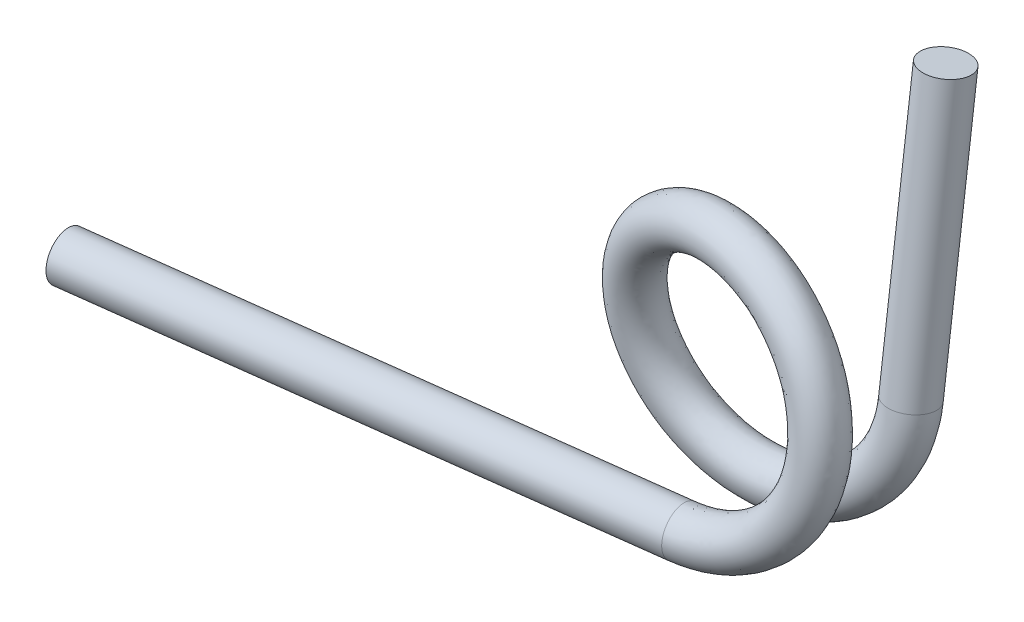
SolidWorks part; units mm, degrees
ref_plane "Front Plane" through (0, 0, 0) normal (0, 0, 1) x (1, 0, 0)
ref_plane "Top Plane" through (0, 0, 0) normal (0, 1, 0) x (1, 0, 0)
ref_plane "Right Plane" through (0, 0, 0) normal (1, 0, 0) x (0, 0, -1)
other "Configuration Table"
sketch "Sketch1" plane through (0, 0, 0) normal (0, 0, 1) x (1, 0, 0)
  circle A0 centre (0, 0) radius 2.5
  dimension "D1" = 5
curve "Helix/Spiral1" pitch 2 height 2.5 turns 1.25
sweep "Sweep1" add path "Helix/Spiral1" circular profile diameter 1 parameters "D3"=1
sketch "Sketch8" plane through (-0.3132, 0, 0.0399) normal (-0.992, 0, 0.1263) x (0.0314, 0.9686, 0.2467)
  circle A1 centre (-1.8049, -3.0237) radius 0.5
  circle A2 centre (-1.8049, -3.0237) radius 0.5
  dimension "D1" = 0
extrude "Boss-Extrude1" add sketch "Sketch8" along normal blind 12
sketch "Sketch9" plane through (0, 0, 0) normal (0, 0.992, -0.1263) x (1, 0, 0)
  circle A1 centre (2.5, 0) radius 0.5
  circle A2 centre (2.5, 0) radius 0.5
  dimension "D1" = 0
extrude "Boss-Extrude2" add sketch "Sketch9" along normal blind 6
